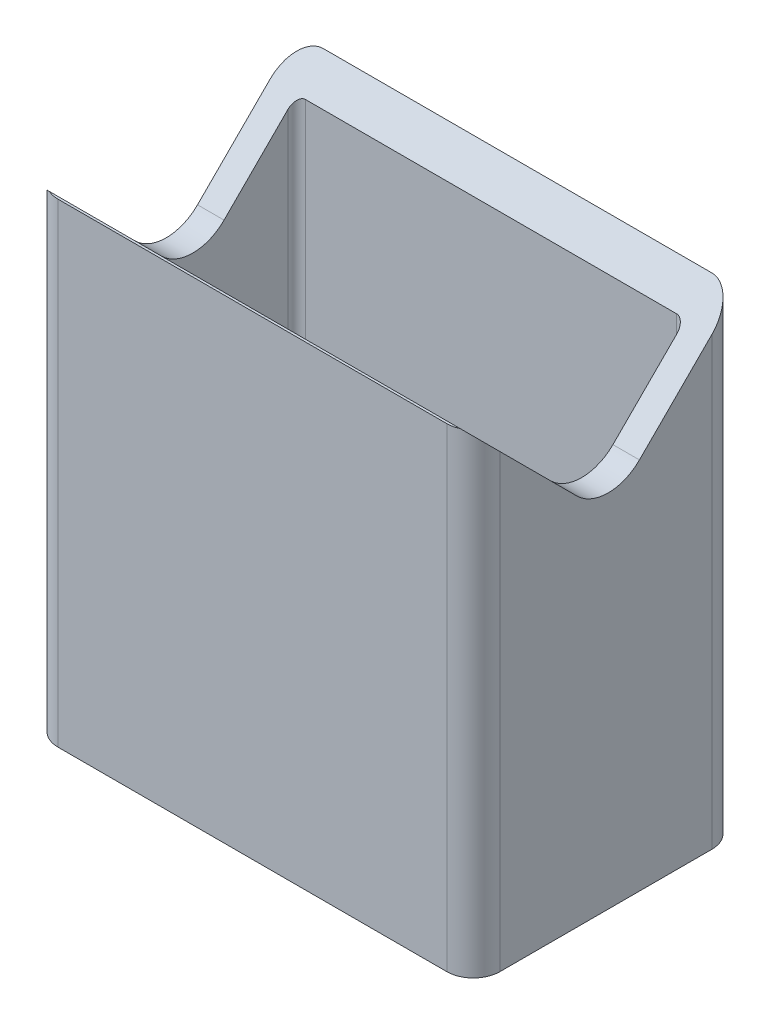
SolidWorks part; units mm, degrees
material "1023 碳钢板 (SS)"
ref_plane "Front Plane" through (0, 0, 0) normal (0, 0, 1) x (1, 0, 0)
ref_plane "Top Plane" through (0, 0, 0) normal (0, 1, 0) x (1, 0, 0)
ref_plane "Right Plane" through (0, 0, 0) normal (1, 0, 0) x (0, 0, -1)
sketch "Sketch1" plane through (0, 0, 0) normal (0, 0, 1) x (1, 0, 0)
  line L1 (-25, 26.85) -> (25, 26.85)
  line L2 (-25, 26.85) -> (-25, -26.85)
  line L3 (-25, -26.85) -> (25, -26.85)
  line L4 (25, 26.85) -> (25, -26.85)
  line L5 (-25, 26.85) -> (25, -26.85) construction
  line L6 (-25, -26.85) -> (25, 26.85) construction
  point P0 (0, 0)
  dimension "D1" = 50
  dimension "D2" = 53.7
extrude "Boss-Extrude1" add sketch "Sketch1" along normal blind 30
shell "Shell1" thickness 3
sketch "Sketch2" plane through (25, 0, 0) normal (1, 0, 0) x (0, 0, -1)
  line L0 (-11.2122, 15.4013) -> (13.5366, 40.15)
  line L5 (-18.2832, 15.4013) -> (-43.032, 40.15)
  line L6 (13.5366, 40.15) -> (-14.7477, 68.4343)
  line L7 (-43.032, 40.15) -> (-14.7477, 68.4343)
  line L8 (-30, 26.85) -> (0, 26.85) construction
  line L9 (-30, -26.85) -> (0, -26.85) construction
  line L10 (-43.032, 40.15) -> (13.5366, 40.15) construction
  arc A0 (-18.2832, 15.4013) -> (-11.2122, 15.4013) centre (-14.7477, 18.9368) ccw
  point P10 (-14.7477, 11.8657)
  dimension "D4" = 5
  dimension "D1" = 40
  dimension "D2" = 40
  dimension "D3" = 67
extrude "Cut-Extrude1" cut sketch "Sketch2" against normal blind 66
fillet "Fillet1" radius 3 4 edges at (-25, -0.1183, 0) (25, -0.1183, 0) (-25, 0, 30) (25, 0, 30)
fillet "Fillet2" radius 1 4 edges at (-22, -1.6183, 3) (22, -1.6183, 3) (-22, -1.366, 27) (22, -1.366, 27)
